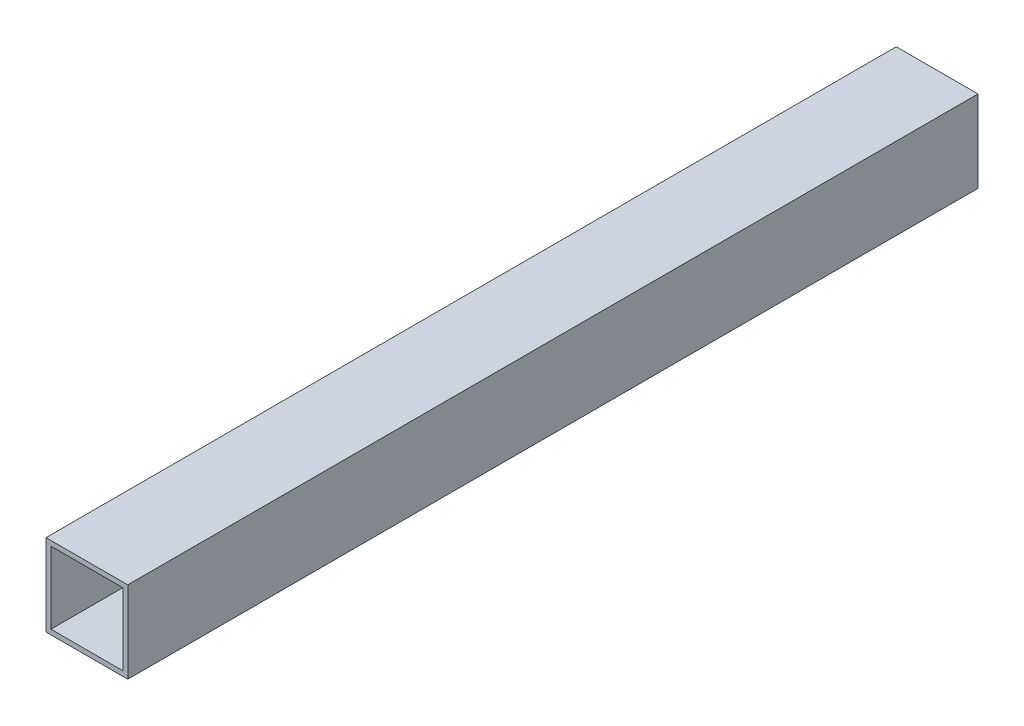
from build123d import *

# Parameters (mm, degrees)
SKETCH_1_W          = 50
SKETCH_1_H          = 50
SKETCH_1_W_2        = 44
SKETCH_1_H_2        = 44
EXTRUDE_1_DEPTH     = 520
SKETCH_2_W          = 50
SKETCH_2_H          = 50
SKETCH_2_W_2        = 44
SKETCH_2_H_2        = 44
EXTRUDE_2_DEPTH     = 70
SKETCH_3_W          = 50
SKETCH_3_H          = 50
CUT_EXTRUDE_1_DEPTH = 70


with BuildPart() as part:
    # 草图1 → 凸台-拉伸1 (new body)
    with BuildSketch(Plane.XY):
        with Locations((25, 25)):
            Rectangle(SKETCH_1_W, SKETCH_1_H)
        with Locations((25, 25)):
            Rectangle(SKETCH_1_W_2, SKETCH_1_H_2, mode=Mode.SUBTRACT)
    extrude(amount=EXTRUDE_1_DEPTH)

    # 草图2 → 凸台-拉伸2 (add)
    with BuildSketch(Plane.XY.offset(520)):
        with Locations((25, 25)):
            Rectangle(SKETCH_2_W, SKETCH_2_H)
        with Locations((25, 25)):
            Rectangle(SKETCH_2_W_2, SKETCH_2_H_2, mode=Mode.SUBTRACT)
    extrude(amount=EXTRUDE_2_DEPTH)

    # 草图3 → 切除-拉伸1 (cut)
    with BuildSketch(Plane.XY.offset(590)):
        with Locations((25, 25)):
            Rectangle(SKETCH_3_W, SKETCH_3_H)
    extrude(amount=-CUT_EXTRUDE_1_DEPTH, mode=Mode.SUBTRACT)


solid = part.part
